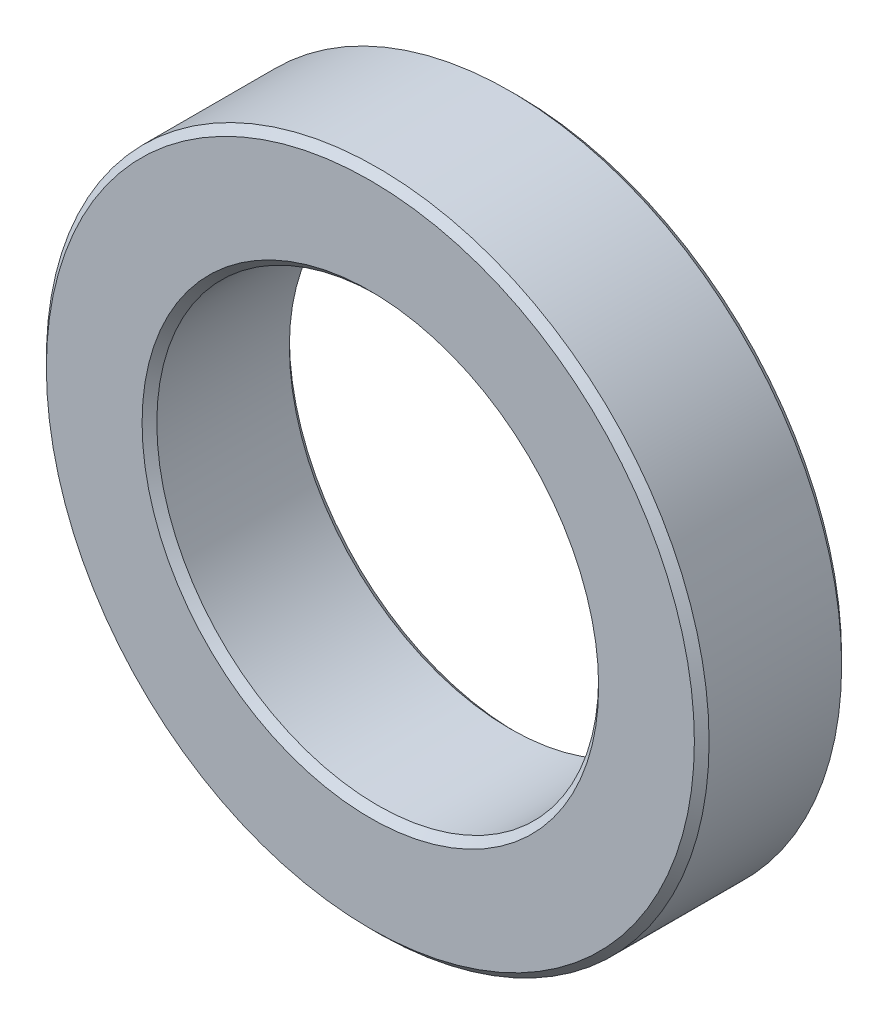
SolidWorks part; units mm, degrees
ref_plane "Front Plane" through (0, 0, 0) normal (0, 0, 1) x (1, 0, 0)
ref_plane "Top Plane" through (0, 0, 0) normal (0, 1, 0) x (1, 0, 0)
ref_plane "Right Plane" through (0, 0, 0) normal (1, 0, 0) x (0, 0, -1)
sketch "Sketch1" plane through (0, 0, 0) normal (0, 0, 1) x (1, 0, 0)
  circle A0 centre (0, 0) radius 15
  circle A1 centre (0, 0) radius 22.5
extrude "Boss-Extrude1" add sketch "Sketch1" along normal blind 10
chamfer "Chamfer1" distance 0.5 angle 45 4 edges at (22.5, 0, 0) (22.5, 0, 10) (15, 0, 0) (15, 0, 10)
